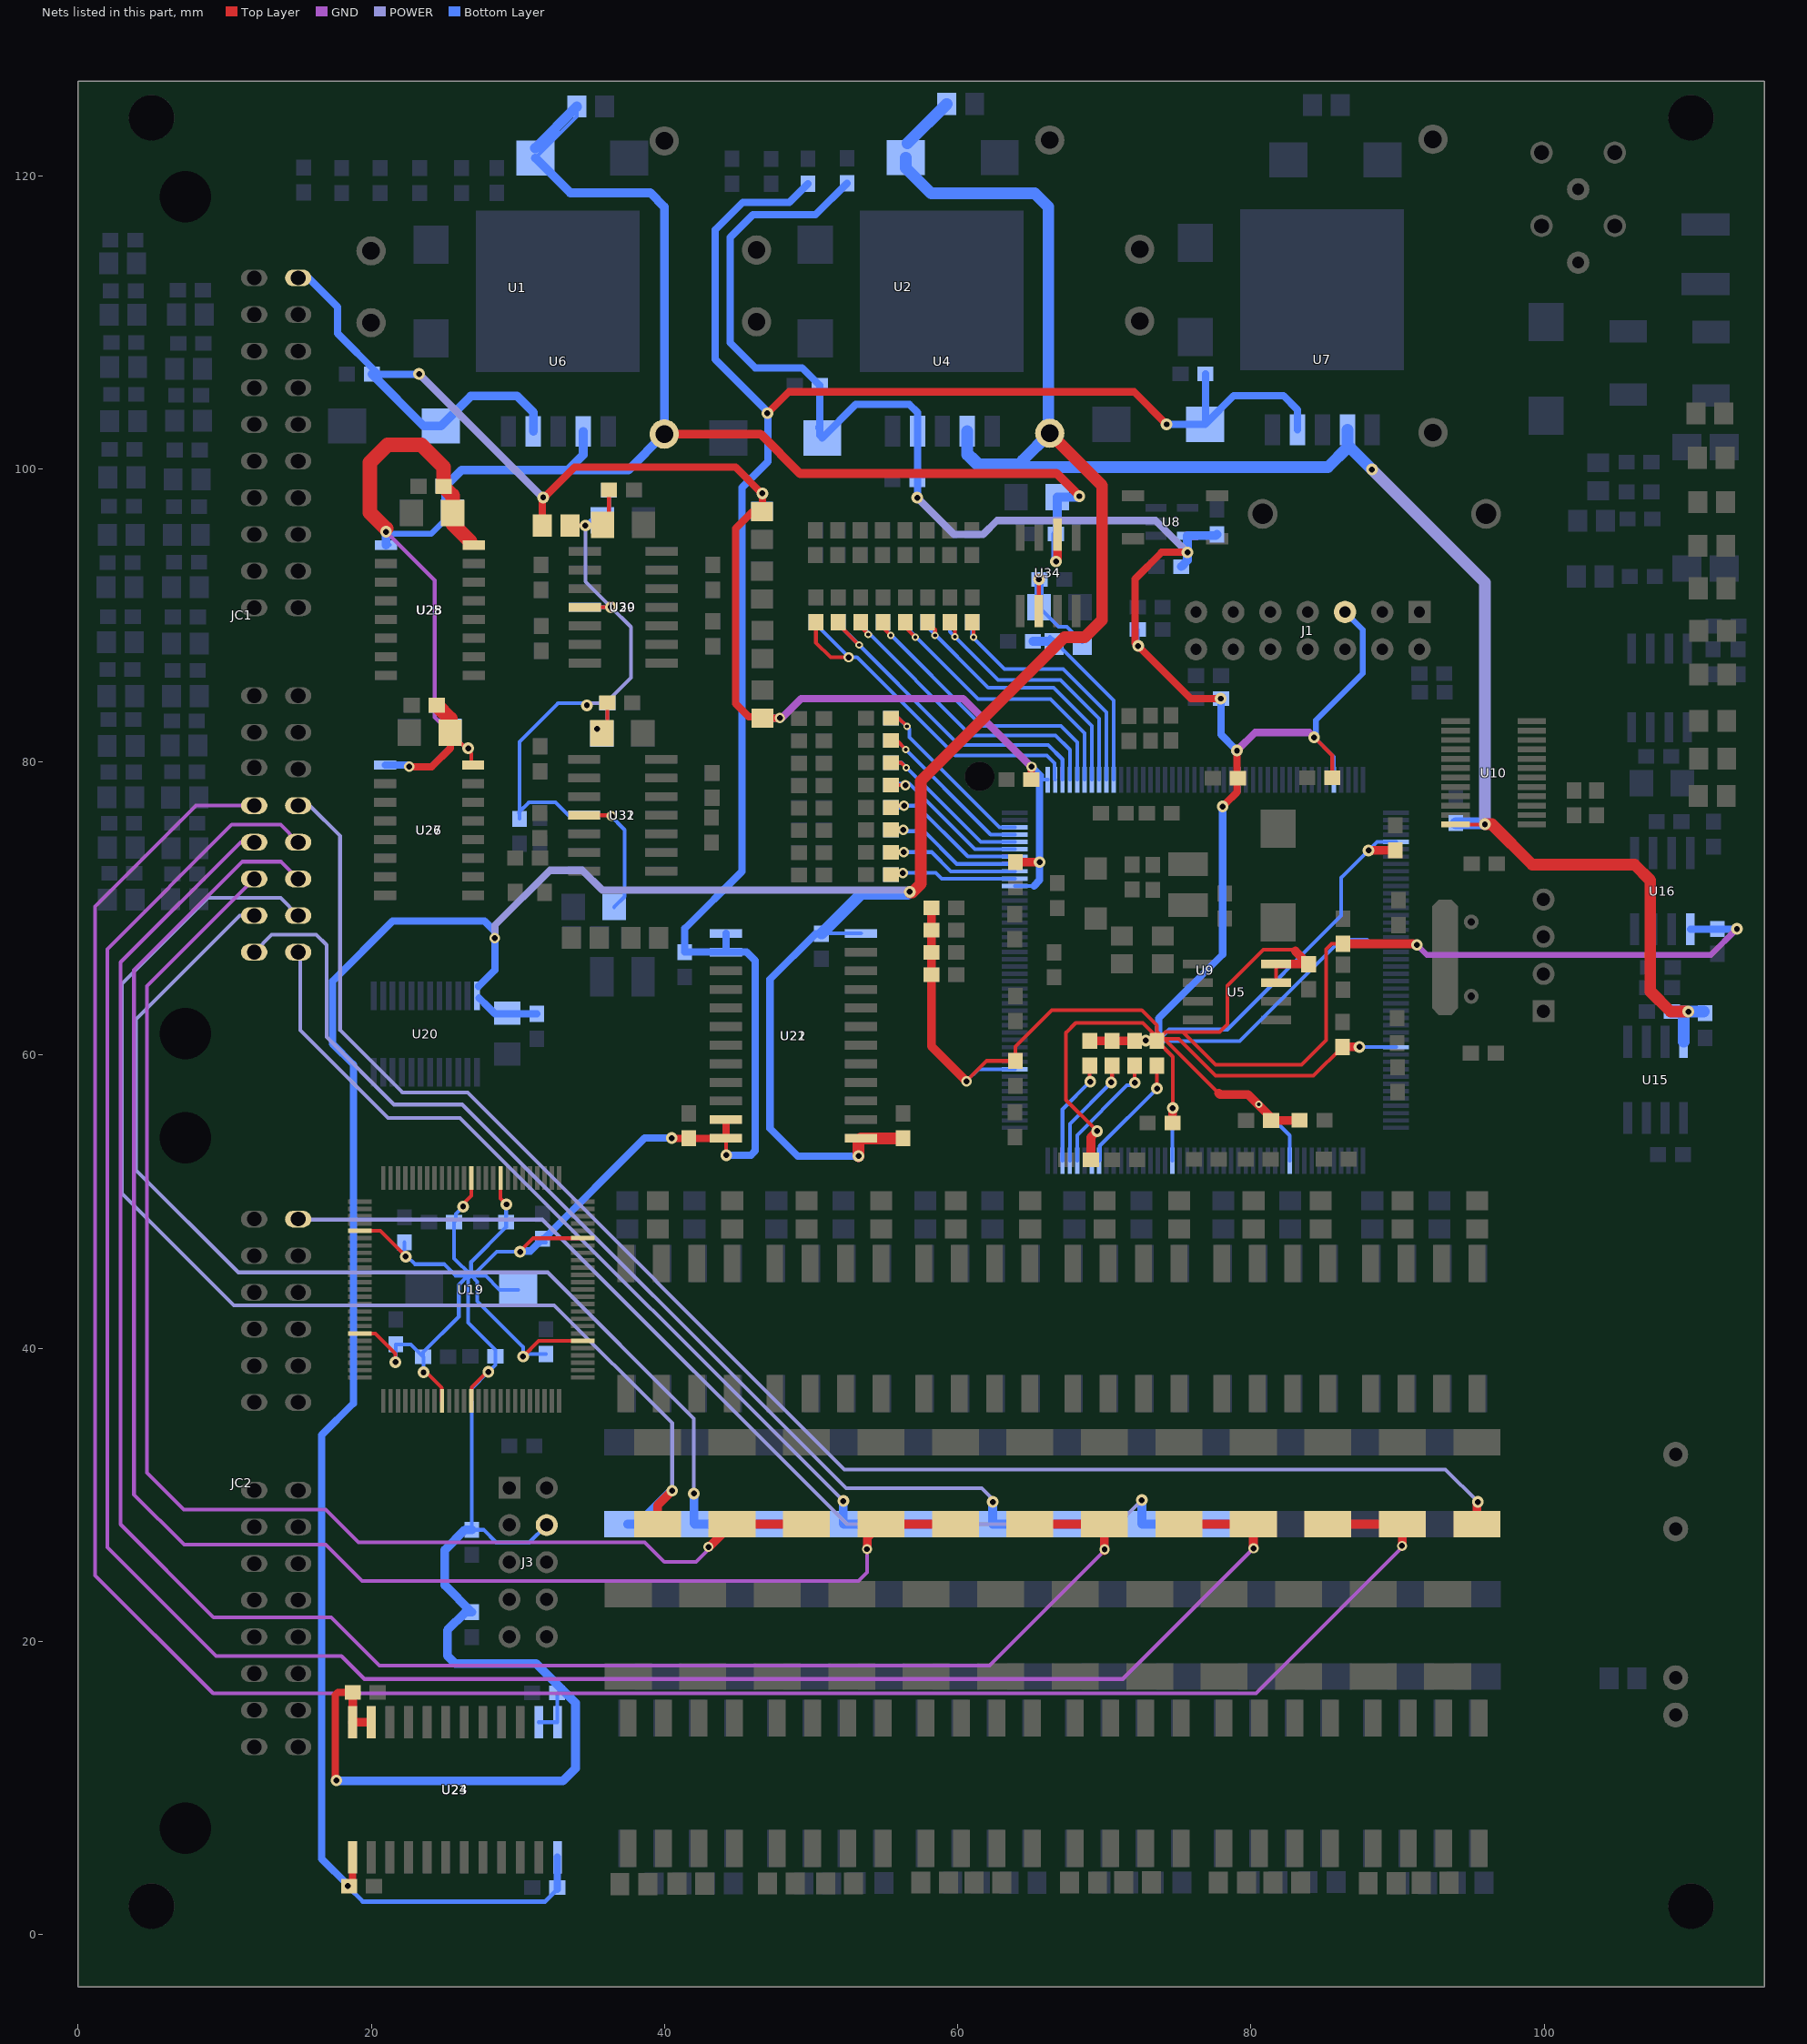
[diagram p0: the nets of this part, all layers, seen from the top]
# Altium PCB MISC86180.PCBDOC (part 4 of 9)
Units mm, origin at the board's own origin, x right, y up, seen from the top; angles counter-clockwise.
Board outline 115 x 130 mm, 4 copper layers (Top Layer, GND, POWER, Bottom Layer); 475 components, 355 nets, 1755 pads, 459 vias.

## Via types
v1: diameter 0.8, hole 0.4, Top Layer to Bottom Layer, 339 vias
v2: diameter 0.7, hole 0.4, Top Layer to Bottom Layer, 83 vias
v3: diameter 0.5, hole 0.254, Top Layer to Bottom Layer, 37 vias

## Nets (pads, with @x,y where several pads share a name; then routed paths per layer and width w, separated by ;. In a path a pad name is that pad's centre, name@x,y a point inside that pad or via, vN(x,y) a via of type N, cw(c..) or ccw(c..) an arc to the next point about the centre after c; other vN are vias at no path point) (continued)
+3.3VA: C15.1 C16.2 C125.2 C127.2 C201.2 C203.2 JC1.1 R131.1 R133.1 R136.1 U6.4 U9.34 U9.45 | length 111.7
  Top Layer w0.254: v1@46.65,98.3 v1(46.67,98.32)
  Top Layer w0.5: R136.1@31.661,96.126 31.661,97.911 33.86,100.11 44.84,100.11 v1@46.65,98.3 ; v1(46.67,98.32) 46.67,97.095 R133.1@46.65,97.075 46.005,97.075 44.85,95.92 44.85,83.97 45.736,83.084 46.604,83.084 R131.1@46.686,83.001 v2@47.949,83.001 ; C203.2@65.02,78.802 65.02,79.6 v2@65.06,79.64
  Top Layer w0.6: C201.2@63.918,73.168 v1(65.582,73.168)
  GND w0.5: v2(47.86,83.01) 47.89,82.98 47.97,82.98 49.31,84.32 60.36,84.32 65.02,79.66 v2@65.06,79.66
  POWER w0.5: v1(23.26,106.47) v1@31.69,98.04
  Bottom Layer w0.254: C127.2@46.65,97.093 46.65,98.3 v1(46.67,98.32) ; v2(47.86,83.01) 47.887,82.983 47.89,82.98 47.97,82.98 v2@47.967,82.983 ; U9.34@63.889,71.543 65.193,71.543 ; 65.582,78.755 65.62,78.793 U9.45@66.139,78.793
  Bottom Layer w0.5: JC1.1@15.01,113.022 15.718,113.022 17.7,111.04 17.7,109.23 20.472,106.458 v1@23.248,106.458 ; C125.2@46.686,82.983 47.887,82.983 v2@47.967,82.983 ; v2(65.03,79.67) 65.62,79.08 65.62,78.793 ; 65.193,71.543 65.582,71.932 v1(65.582,73.168) 65.582,78.755
  Bottom Layer w0.6: C16.2@20.04,106.458 23.576,102.922 C15.1@24.744,102.922 26.792,104.97 29.94,104.97 31.047,103.863 U6.4@31.047,102.555
  other v1: 31.72,98.04
+3.3VD: C11.1 C12.2 C19.2 C20.2 C21.2 C22.2 C23.2 C24.2 C25.2 C26.2 C27.2 C28.2 C29.2 C68.2 J1.5 R1.1 R2.1 R6.1 R7.1 R8.2 R9.2 R10.2 R11.2 R12.2 R86.1 R88.1 R90.1 R92.1 R94.1 U4.4 U5.3 U5.4 U8.5 U9.9 U9.71 U9.84 U9.93 U9.107 U9.121 U9.143 U9.159 U9.170 U16.1 | length 356.9
  Top Layer w0.254: v2(60.59,58.22) 61.98,59.61 C27.2@63.928,59.61 63.928,60.578 66.41,63.06 72.54,63.06 73.57,62.03 73.57,61.62 77.795,57.395 ; v1@69.39,54.71 v1(69.5,54.82) 67.38,56.94 67.38,61.53 68.04,62.19 72.61,62.19 R12.2@73.57,61.23 ; R10.2@70.522,60.976 R11.2@72.046,60.976 ; C20.2@74.64,55.372 C20.2@74.66,55.392 ; v1(74.66,56.39) 74.66,59.886 R12.2@73.57,60.976 73.582,60.988 R12.2@73.714,61.12 ; v1(79.04,80.78) v1@79.1,80.72 ; C22.2@81.36,55.542 81.36,55.56 C22.2@81.36,55.59 ; U5.3@81.713,64.94 U5.4@81.713,66.21 ; 83.024,67.104 82.938,67.19 80.83,67.19 78.38,64.74 78.38,62.1 77.85,61.57 75.35,61.57 ; R8.2@83.304,55.542 R8.2@83.31,55.548 ; C26.2@83.928,66.2 83.918,66.21 C26.2@84.1,66.21 ; v1(84.3,81.68) 85.54,80.44 C29.2@85.54,78.922 85.563,78.922 C29.2@85.64,78.999 ; C23.2@86.232,60.56 84.262,58.59 77.59,58.59 75.06,61.12 R12.2@73.714,61.12 ; C24.2@86.342,67.52 C24.2@86.262,67.6 85.49,67.6 85.12,67.23 85.12,61.02 83.44,59.34 77.58,59.34 75.35,61.57 ; v1@88.02,73.98 v1@88.15,73.98 ; v1@91.15,67.52 v1(91.31,67.52) ; R12.2@73.714,61.12 74.164,61.57 75.35,61.57 ; v1(78.06,76.96) 78.22,77.12 78.4,77.12 78.24,76.96 v1(78.06,76.96)
  Top Layer w0.5: v1(75.662,94.3) 73.9,94.3 72.09,92.49 72.09,88.12 v1(72.3,87.91) 75.888,84.322 v1(77.932,84.322) ; v1@78.22,77.12 79.04,77.94 v1(79.04,80.78)
  Top Layer w0.6: R92.1@58.2,70.054 R90.1@58.2,68.53 R88.1@58.2,67.006 R86.1@58.2,65.482 58.2,60.61 v2(60.59,58.22) ; R9.2@68.998,60.976 R10.2@70.522,60.976 R11.2@72.046,60.976 R12.2@73.57,60.976 ; C25.2@69.08,52.862 69.08,54.4 v1@69.39,54.71 ; C20.2@74.64,55.372 74.64,56.37 v1(74.66,56.39) ; 77.795,57.395 77.87,57.32 79.78,57.32 81.36,55.74 C22.2@81.36,55.59 ; C22.2@81.36,55.542 R8.2@83.304,55.542 ; U5.4@81.713,66.21 83.918,66.21 83.024,67.104 ; C23.2@86.232,60.56 v1(87.39,60.56) ; C24.2@86.262,67.6 91.07,67.6 v1@91.15,67.52 ; v1@88.15,73.98 C21.2@89.832,73.98
  GND w0.254: v1(79.04,80.78) 79.06,80.78 79.14,80.86 79.14,80.88 v1@79.14,80.93 ; v1@84.11,81.56 84.18,81.56 v1(84.3,81.68)
  GND w0.4: v1(91.31,67.52) 92,66.83 111.35,66.83 v1(113.14,68.62)
  GND w0.5: v1(79.04,80.78) 79.14,80.88 80.27,82.01 83.97,82.01 v1(84.3,81.68)
  POWER w0.5: v1(57.23,98.03) 59.74,95.52 61.726,95.52 62.676,96.47 73.492,96.47 v1(75.662,94.3)
  Bottom Layer w0.254: C11.1@50.404,102.742 C11.1@50.404,102.88 ; C11.1@50.58,102.276 C11.1@50.754,102.102 52.98,104.328 ; v2(60.59,58.22) 61.413,59.043 U9.9@63.889,59.043 ; U9.170@69.139,52.793 69.139,54.459 v1(69.5,54.82) ; v1@72.272,87.938 R6.1@72.272,89.032 ; 73.725,61.14 73.725,61.055 ; U9.159@74.639,52.793 v1@74.639,56.369 ; v1(77.932,84.322) R7.1@77.95,84.322 ; v1@78.894,80.714 79.139,80.469 U9.71@79.139,78.793 ; v3(80.52,56.64) 82.639,54.521 U9.143@82.639,52.793 ; v1@84.43,81.55 85.639,80.341 U9.84@85.639,78.793 U9.84@85.65,78.783 ; v1(87.39,60.56) 87.407,60.543 U9.121@89.889,60.543 ; U9.93@89.889,74.543 88.583,74.543 v1(88.01,73.97) 86.15,72.11 86.15,69.52 78.38,61.75 74.42,61.75 73.725,61.055 ; v1@91.287,67.543 U9.107@89.889,67.543 88.247,67.543 87.92,67.87 86.15,67.87 79.23,60.95 73.62,60.95 73.725,61.055
  Bottom Layer w0.4: v1@84.43,81.55 84.43,82.85 87.62,86.04 87.62,89.019 J1.5@86.406,90.233
  Bottom Layer w0.5: C11.1@50.58,102.276 C12.2@50.58,105.688 49.378,106.89 46.18,106.89 44.47,108.6 44.47,115.78 46.02,117.33 50.29,117.33 R94.1@52.442,119.482 ; C11.1@50.754,102.102 53.042,104.39 56.687,104.39 57.247,103.83 U4.4@57.247,102.565 v1@57.247,98.047 ; 73.725,61.14 73.69,61.175 73.69,62.5 78.06,66.87 v1(78.06,76.96) ; R7.1@77.95,84.322 77.95,81.87 78.894,80.926 v1@78.894,80.714 ; U16.1@109.963,68.591 v1@113.111,68.591
  Bottom Layer w0.6: v1(72.82,61) 73.515,61 73.69,61.175 ; R2.1@75.24,93.332 75.662,93.754 v1(75.662,94.3) U8.5@75.662,95.435 77.581,95.435 C19.2@77.672,95.526
+3.3VD2: C17.1 C18.2 C81.1 C82.2 C83.2 C84.2 C85.2 C86.2 C87.2 C88.2 C89.2 C92.2 C93.2 C94.2 C95.2 J3.4 R84.1 R85.1 R95.1 U7.4 U19.9 U19.13 U19.31 U19.45 U19.59 U19.63 U19.80 U19.94 U21.23 U21.24 U22.23 U22.24 U23.23 U23.24 U24.23 U24.24 | length 297.7
  Top Layer w0.254: v1@17.54,10.6 v1@17.54,10.735 ; v1@17.605,10.535 v1(17.62,10.52) ; 17.605,16.415 17.605,16.445 ; U23.24@18.719,14.492 U23.24@18.73,14.503 ; U19.94@19.216,41.014 20.276,41.014 21.64,39.65 v1(21.64,39.06) ; U19.80@19.216,48.014 20.606,48.014 22.34,46.28 v1(22.34,46.26) ; v1(23.56,38.36) 23.751,38.36 24.81,37.301 24.81,36.42 U19.9@24.816,36.414 ; v1(26.26,49.67) 26.1,49.67 26.092,49.678 26.092,49.68 26.816,50.404 U19.63@26.816,51.614 ; U19.13@26.816,36.414 26.861,36.459 26.861,37.34 27.911,38.39 v1(27.98,38.39) ; U19.59@28.816,51.614 28.816,50.214 v1(29.21,49.82) ; v1(30.15,46.58) 30.15,46.63 31.03,47.51 34.412,47.51 U19.45@34.416,47.514 ; v1(30.35,39.44) 31.42,40.51 34.412,40.51 U19.31@34.416,40.514 ; U22.24@44.192,54.329 U22.24@44.192,54.329 v1@44.192,53.198
  Top Layer w0.5: v1@17.54,10.6 v1@17.605,10.535 ; v1@17.54,10.735 17.54,16.35 17.605,16.415 17.718,16.528 C94.2@18.73,16.528 ; v1@40.5,54.33 C92.2@41.662,54.33 U22.24@44.192,54.329 ; U22.24@44.192,54.329 U22.23@44.192,55.599 ; v1(47.01,103.79) 48.47,105.25 72.02,105.25 v1(74.238,103.032)
  Top Layer w0.6: U23.24@18.719,14.492 U23.23@19.989,14.492 ; U23.24@18.73,14.503 C94.2@18.73,16.528
  Bottom Layer w0.254: v1(17.62,10.52) v1@17.69,10.59 ; v1(21.64,39.06) 21.658,39.078 C86.2@21.658,40.27 22.682,40.27 C88.2@23.53,39.422 ; C87.2@22.262,47.228 22.262,46.338 v1(22.34,46.26) 22.45,46.26 22.97,45.74 24.97,45.74 25.745,44.965 26.61,44.965 25.965,44.32 25.965,42.165 23.53,39.73 C88.2@23.53,39.422 ; v1(23.56,38.36) 23.56,39.392 C88.2@23.53,39.422 ; v1(26.26,49.67) 25.76,49.17 25.76,48.73 C89.2@25.634,48.604 25.634,46.136 26.805,44.965 ; v1(29.21,49.82) 29.19,49.8 C82.2@29.19,48.604 29.19,48.28 26.805,45.895 26.805,44.965 ; C81.1@30.01,43.996 28.75,43.996 27.781,44.965 26.95,44.965 ; v1@30.21,46.64 v1(30.15,46.58) 28.565,46.58 26.95,44.965 ; U24.23@31.419,14.492 U24.24@32.689,14.492 ; C84.2@31.678,47.228 C84.2@31.914,47.228 ; C84.2@31.678,47.47 C84.2@31.77,47.47 ; C85.2@31.914,39.608 30.518,39.608 v1(30.35,39.44) 30.35,40.09 27.22,43.22 27.22,44.55 26.805,44.965 ; J3.4@31.965,27.945 30.769,26.75 28.53,26.75 27.66,27.62 R84.1@26.848,27.62 26.848,37.258 v1(27.98,38.39) 28.46,38.87 C83.2@28.46,39.448 28.46,39.89 26.61,41.74 26.61,44.77 26.805,44.965 ; U24.24@32.66,14.521 U24.24@32.689,14.492 ; C95.2@32.689,16.459 U24.24@32.689,14.492 ; v1(44.21,53.18) v1@44.36,53.18 ; 26.805,44.965 26.95,44.965
  Bottom Layer w0.5: v1@30.04,46.64 30.21,46.64 30.848,46.64 C84.2@31.678,47.47 ; C84.2@31.77,47.47 38.64,54.34 v1(40.49,54.34) ; U21.23@44.192,67.029 C93.2@41.382,67.03 41.382,68.642 45.27,72.53 45.27,98.71 47.05,100.49 47.05,103.86 43.45,107.46 43.45,116.3 45.33,118.18 48.516,118.18 R95.1@49.788,119.452 ; U21.24@44.192,68.299 U21.23@44.192,67.029 45.591,67.029 46.18,66.44 46.18,53.47 45.89,53.18 v1@44.36,53.18 ; v1(74.238,103.032) C17.1@76.864,103.032 C17.1@76.89,103.058 ; C18.2@76.89,106.468 C17.1@76.89,103.058 ; U7.4@83.167,102.665 83.167,104.033 82.2,105 78.832,105 C17.1@76.89,103.058
  Bottom Layer w0.6: v1(17.62,10.52) 17.64,10.5 33.08,10.5 33.92,11.34 33.92,15.81 31.23,18.5 25.71,18.5 25.18,19.03 25.18,20.77 26.41,22 R85.1@26.848,22 25.01,23.838 25.01,26.24 26.39,27.62 R84.1@26.848,27.62
+5V: C6.1 C7.2 C57.2 C67.2 C90.2 C91.2 C96.2 C97.2 C98.2 C99.2 R21.2 U2.3 U4.2 U7.2 U10.24 U15.8 U20.24 U21.1 U22.1 U23.1 U24.1 | length 340.5
  Top Layer w0.254: v1(53.23,53.11) v1@53.392,53.272 ; 53.392,54.02 U22.1@53.392,54.329 ; U10.24@93.946,75.738 v1@95.938,75.738
  Top Layer w0.5: C98.2@18.48,3.308 18.725,3.553 U23.1@18.725,5.28
  Top Layer w0.8: v1(53.23,53.11) 53.23,54.02 ; U22.1@53.392,54.329 C96.2@56.272,54.33 ; v1(56.72,71.14) 56.77,71.09 56.88,71.09 57.474,71.684 57.474,78.704 67.277,88.507 68.653,88.507 69.84,89.694 69.84,98.858 U2.3@66.271,102.428 ; v1(95.95,75.75) 96.43,75.75 99.18,73 106.154,73 107.23,71.924 107.23,66.02 107.23,64.35 108.612,62.968 v1(109.83,62.968)
  POWER w0.254: v2(28.42,67.99) v2@28.42,68.18
  POWER w0.5: v2@28.42,68.18 28.42,68.85 32.18,72.61 34.4,72.61 35.75,71.26 56.47,71.26 56.637,71.093 56.673,71.093 v1(56.72,71.14)
  POWER w0.8: v1(88.25,99.95) 95.95,92.25 v1(95.95,75.75)
  Bottom Layer w0.254: C90.2@31.237,62.867 C90.2@31.288,62.816 ; C97.2@50.692,68.28 50.711,68.299 U21.1@53.392,68.299 ; C6.1@56.456,121.228 C6.1@56.559,121.331 ; 60.647,101.463 61.53,100.58 64.423,100.58 ; U2.3@66.25,102.522 66.25,102.448 U2.3@66.271,102.428 ; 86.407,101.597 86.567,101.757 U7.2@86.567,101.633 ; v1@95.87,75.83 v1(95.95,75.75) ; R21.2@110.874,62.968 R21.2@110.972,62.87
  Bottom Layer w0.3: v1@18.4,3.27 19.412,2.258 31.858,2.258 C99.2@32.68,3.08
  Bottom Layer w0.5: v1@18.4,3.27 v1(18.4,3.33) 18.4,3.39 16.62,5.17 16.62,34.09 18.77,36.24 18.77,59.36 17.36,60.77 17.36,65.04 21.46,69.14 27.72,69.14 28.42,68.44 v2(28.42,67.99) 28.42,65.8 27.32,64.7 U20.24@27.32,64.68 ; U20.24@27.36,63.889 27.97,63.28 28.129,63.12 28.433,62.816 C90.2@31.288,62.816 ; C99.2@32.68,3.08 C99.2@32.68,3.208 ; C99.2@32.68,3.228 32.68,5.283 U24.1@32.689,5.292 ; C97.2@50.692,68.28 50.3,68.28 47.19,65.17 47.19,55 49.08,53.11 v1(53.23,53.11)
  Bottom Layer w0.8: C97.2@50.711,68.299 53.422,71.01 56.59,71.01 v1(56.72,71.14) ; C6.1@56.456,121.228 56.456,120.514 58.18,118.79 65.25,118.79 66.176,117.864 U2.3@66.176,102.522 ; C6.1@56.559,122.2 C7.2@59.251,124.892 ; U4.2@60.647,102.565 60.647,101.463 60.647,100.953 61.49,100.11 85.24,100.11 86.567,101.437 86.567,101.633 v1(88.25,99.95) ; 64.423,100.58 U2.3@66.271,102.428 ; U7.2@86.567,101.757 U7.2@86.567,102.665 ; C57.2@93.968,75.83 v1@95.87,75.83 ; C67.2@108.7,62.968 v1(109.83,62.968) R21.2@110.874,62.968 ; U15.8@109.501,60.913 109.501,62.64
+5VA: C3.1 C4.2 C129.2 C130.2 C131.2 C140.2 C141.2 C142.2 C143.2 C144.2 C205.2 C206.2 U1.3 U6.2 U25.16 U26.16 U27.16 U28.16 U34.2 | length 153.7
  Top Layer w0.254: v2@22.5,79.651 v2@22.639,79.79 ; C141.2@24.77,83.75 C141.2@24.77,83.87 ; C129.2@24.92,97.611 C129.2@25.539,96.992 C129.2@25.539,96.251 ; C130.2@25.381,81.34 C130.2@25.381,82.006 26.81,80.577 26.81,79.911 U27.16@26.934,79.787 ; v1(66.7,93.68) v1@66.735,93.715
  Top Layer w0.5: v2(22.58,79.68) 24.12,79.68 25.381,80.941 C130.2@25.381,82.006
  Top Layer w0.6: U1.3@39.981,102.368 46.544,102.368 49.232,99.68 66.74,99.68 v1(68.29,98.13) ; v1@66.735,93.715 66.793,93.773 U34.2@66.793,95.507
  Top Layer w1: v1@21,95.917 19.91,97.007 19.91,100.43 21.12,101.64 23.4,101.64 24.92,100.12 C140.2@24.92,98.798 25.539,98.179 C129.2@25.539,96.992 25.539,96.251 U25.16@26.735,95.055 ; C141.2@24.46,83.872 25.381,82.951 C130.2@25.381,82.006
  GND w0.254: v1(21,95.7) 24.32,92.38 24.32,83.06 26.45,80.93 v1(26.61,80.93)
  Bottom Layer w0.254: U28.16@20.998,94.797 U28.16@21.257,94.797 ; v1@20.998,95.548 v1@21,95.55 ; v1@21.06,95.61 v1@21,95.55 ; v1@21.14,95.56 v1(21,95.7) v1@21,95.55 ; v2@22.58,79.79 22.63,79.79 24.05,79.79 25.381,81.121 C143.2@25.381,82.042 ; C143.2@24.77,82.653 C144.2@24.77,83.906 ; C3.1@31.186,121.208 34.021,124.043 C4.2@34.021,124.712 ; v1@66.69,93.69 v1(66.7,93.68) ; C205.2@66.779,98.068 C205.2@66.841,98.13 ; v1@68.228,98.13 v1(68.29,98.13)
  Bottom Layer w0.4: v1@21.14,95.56 24.081,95.56 C131.2@25.529,97.008
  Bottom Layer w0.5: U26.16@20.941,79.79 v2@22.58,79.79
  Bottom Layer w0.6: U28.16@20.998,94.797 20.998,95.548 v1@20.998,95.698 ; C131.2@25.529,97.008 25.074,97.463 25.074,98.834 26.148,99.908 33.398,99.908 ; C3.1@31.186,121.208 33.574,118.82 39.03,118.82 39.981,117.869 U1.3@39.981,102.368 37.522,99.908 33.398,99.908 ; U6.2@34.447,102.555 34.447,100.957 33.398,99.908 ; v1@66.69,93.69 C206.2@66.69,95.548 66.779,95.637 C205.2@66.779,98.068 v1@68.228,98.068
  Bottom Layer w0.7: C3.1@31.186,121.877 C4.2@34.021,124.712
+OPV: C132.2 C133.2 C134.2 C135.2 C136.2 C137.2 C138.2 C139.2 C208.2 C209.2 R136.2 U29.4 U30.4 U31.4 U32.4 | length 60.4
  Top Layer w0.254: R136.2@33.561,96.126 35.728,96.126 C132.2@35.765,96.162 36.204,96.601 C136.2@36.204,98.564 ; U31.4@34.514,76.365 36.325,76.365 v2(36.38,76.31) ; U29.4@34.554,90.551 v1@36.321,90.551 ; C134.2@35.725,81.976 36.094,82.345 C138.2@36.094,84.048
  POWER w0.254: v1(34.6,96.13) 34.6,92.31 v1(36.34,90.57) 37.7,89.21 37.7,85.76 35.96,84.02 34.83,84.02 34.7,83.89 v1(34.7,83.86)
  Bottom Layer w0.254: C209.2@30.092,76.5 30.092,76.585 30.747,77.24 32.55,77.24 33.415,76.375 U32.4@34.514,76.375 36.275,76.375 37.28,75.37 37.28,70.809 C208.2@36.569,70.098 ; C209.2@30.102,76.12 30.102,81.382 32.732,84.012 C139.2@36.094,84.012 36.094,82.309 C135.2@35.725,81.94 v1(35.4,82.265) ; U30.4@34.554,90.561 36.331,90.561 v1(36.34,90.57) ; v1(34.6,96.13) 34.952,96.482 C133.2@35.761,96.482 36.204,96.925 C137.2@36.204,98.528
A1_12: R12.1 U9.169 | length 8.1
  Top Layer w0.254: v1@73.57,57.73 R12.1@73.57,59.276
  Bottom Layer w0.254: U9.169@69.639,52.793 69.684,52.839 69.684,53.809 73.58,57.704 v1(73.58,57.72)
A1_13: R11.1 U9.172 | length 8.6
  Top Layer w0.254: v1@72.046,57.946 R11.1@72.046,59.276
  Bottom Layer w0.254: U9.172@68.139,52.793 68.139,54.539 71.54,57.94 72.04,57.94 72.07,57.97 v1(72.07,58.12)
A1_14: R10.1 U9.173 | length 7.8
  Top Layer w0.254: v1@70.522,57.982 R10.1@70.522,59.276
  Bottom Layer w0.254: U9.173@67.639,52.793 67.639,55.319 v1(70.46,58.14)
A1_15: R9.1 U9.174 | length 7.2
  Top Layer w0.254: v1@68.998,58.222 R9.1@68.998,59.276
  Bottom Layer w0.254: U9.174@67.139,52.793 67.139,56.299 v1(69.03,58.19)
AD_REF: C195.2 C196.2 R180.2 U34.6 | length 8
  Top Layer w0.254: U34.6@65.523,90.307 65.523,92.443 v1(65.53,92.45)
  Bottom Layer w0.254: C195.2@65.57,90.581 C195.2@65.541,90.552 66.877,89.215 67.422,89.215 R180.2@68.479,88.158 ; C196.2@65.57,92.413 C196.2@65.57,92.442
  Bottom Layer w0.6: C195.2@65.541,90.552 C196.2@65.541,92.413
AD_REFIN: C197.2 R180.1 U9.54 | length 12.8
  Bottom Layer w0.254: C197.2@65.107,88.12 C197.2@65.13,88.12 ; R180.1@66.292,88.538 70.639,84.191 U9.54@70.639,78.793
  Bottom Layer w0.6: C197.2@65.13,88.228 R180.1@66.389,88.228
ADCINA0: C171.2 R154.1 U9.42 | length 13.2
  Top Layer w0.254: R154.1@55.468,82.988 R154.1@55.44,82.988 55.962,82.988 v3(56.53,82.42)
  Bottom Layer w0.254: C171.2@55.44,82.988 55.952,82.988 56.7,82.24 56.7,81.69 62.847,75.543 U9.42@63.889,75.543
ADCINA1: C174.2 R156.1 U9.41 | length 12.5
  Top Layer w0.254: R156.1@55.536,81.464 R156.1@55.44,81.464 55.846,81.464 v3(56.46,80.85)
  Bottom Layer w0.254: C174.2@55.44,81.464 55.816,81.464 62.237,75.043 U9.41@63.889,75.043
ADCINA2: C177.2 R158.1 U9.40 | length 11.9
  Top Layer w0.254: R158.1@55.44,79.94 56.13,79.94 v3(56.47,79.6)
  Bottom Layer w0.254: C177.2@55.44,79.94 56.18,79.94 61.577,74.543 U9.40@63.889,74.543
ADCINA3: C180.2 R160.1 U9.39 | length 11.4
  Top Layer w0.254: R160.1@55.44,78.416 v2(56.424,78.416)
  GND w0.254: v2(56.424,78.416) v2@56.47,78.37
  Bottom Layer w0.254: C180.2@55.44,78.416 55.544,78.52 56.7,78.52 61.177,74.043 U9.39@63.889,74.043
ADCINA4: C183.2 R162.1 U9.38 | length 10.9
  Top Layer w0.254: R162.1@55.44,76.892 55.56,77.012 v2(56.33,77.012)
  Bottom Layer w0.254: C183.2@55.44,76.892 56.21,76.892 v2(56.33,77.012) 57.218,77.012 60.687,73.543 U9.38@63.889,73.543
ADCINA5: C186.2 R164.1 U9.37 | length 10.1
  Top Layer w0.254: R164.1@55.44,75.368 v2(56.282,75.368)
  Bottom Layer w0.254: C186.2@55.528,75.28 57.7,75.28 59.937,73.043 U9.37@63.889,73.043
ADCINA6: C189.2 R166.1 U9.36 | length 9.9
  Top Layer w0.254: R166.1@55.44,73.844 56.304,73.844 v2(56.31,73.85)
  Bottom Layer w0.254: C189.2@55.44,73.844 56.304,73.844 v2(56.31,73.85) 58.22,73.85 59.527,72.543 U9.36@63.889,72.543
ADCINA7: C192.2 R168.1 U9.35 | length 9.5
  Top Layer w0.254: R168.1@55.44,72.32 56.14,72.32 v2(56.25,72.43)
  Bottom Layer w0.254: C192.2@55.44,72.32 C192.2@55.47,72.29 ; C192.2@55.44,72.43 58.51,72.43 58.897,72.043 U9.35@63.889,72.043
ADCINB0: C147.2 R138.1 U9.46 | length 25.5
  Top Layer w0.254: R138.1@50.32,89.532 50.32,88.14 51.32,87.14 v2(52.55,87.14)
  Bottom Layer w0.254: C147.2@50.32,89.532 50.32,89.402 52.569,87.153 53.117,87.153 59.82,80.45 66.06,80.45 66.594,79.916 66.594,78.839 U9.46@66.639,78.793
ADCINB1: C150.2 R140.1 U9.47 | length 22.8
  Top Layer w0.254: R140.1@51.844,89.532 51.844,89.402 53.266,87.98 v3(53.27,87.98)
  Bottom Layer w0.254: C150.2@51.844,89.532 51.844,89.406 60.09,81.16 66.16,81.16 67.139,80.181 U9.47@67.139,78.793
ADCINB2: C153.2 R142.1 U9.48 | length 21.1
  Top Layer w0.254: R142.1@53.368,89.532 53.368,89.232 53.9,88.7 v3(53.89,88.69)
  Top Layer w0.6: R142.1@53.368,89.468 R142.1@53.368,89.532
  Bottom Layer w0.254: C153.2@53.368,89.532 53.368,89.352 60.9,81.82 66.65,81.82 67.639,80.831 U9.48@67.639,78.793
ADCINB3: C156.2 R144.1 U9.49 | length 20.5
  Top Layer w0.254: R144.1@54.892,89.532 54.892,89.168 v3(55.43,88.63)
  Bottom Layer w0.254: C156.2@54.892,89.532 54.892,89.208 61.64,82.46 67.02,82.46 68.139,81.341 U9.49@68.139,78.793
ADCINB4: C159.2 R146.1 U9.50 | length 20
  Top Layer w0.254: R146.1@56.416,89.528 R146.1@56.416,89.532 56.416,89.194 v3(57.1,88.51)
  Top Layer w0.6: R146.1@56.414,89.53 R146.1@56.416,89.532
  Bottom Layer w0.254: C159.2@56.416,89.532 56.416,89.254 v3@57.12,88.55 ; v3@57.11,88.56 v3@57.12,88.55 ; U9.50@68.639,78.793 68.639,81.971 66.32,84.29 61.38,84.29 v3@57.12,88.55
ADCINB5: C162.2 R148.1 U9.51 | length 19.1
  Top Layer w0.254: R148.1@57.94,89.532 58.45,89.022 v3(58.45,88.63)
  Bottom Layer w0.254: C162.2@57.94,89.532 57.94,89.21 62.08,85.07 66.54,85.07 69.139,82.471 U9.51@69.139,78.793
ADCINB6: C165.2 R150.1 U9.52 | length 18.6
  Top Layer w0.254: R150.1@59.464,89.532 59.81,89.186 v3(59.81,88.54)
  Top Layer w0.6: R150.1@59.464,89.532 R150.1@59.464,89.564
  Bottom Layer w0.254: C165.2@59.464,89.532 59.464,88.896 62.76,85.6 67,85.6 69.639,82.961 U9.52@69.639,78.793
ADCINB7: C168.2 R152.1 U9.53 | length 18
  Top Layer w0.254: R152.1@60.988,89.532 61.08,89.44 v3(61.08,88.51)
  Top Layer w0.6: R152.1@60.988,89.482 R152.1@60.988,89.532
  Bottom Layer w0.254: C168.2@60.988,89.532 60.988,88.542 63.18,86.35 67.19,86.35 70.139,83.401 U9.53@70.139,78.793
  Bottom Layer w0.6: C168.2@60.966,89.51 C168.2@60.988,89.532
BAT1: F1.1 JC1.24 | length 109.4
  Top Layer w0.6: F1.1@95.396,28.006 95.396,29.446 v1(95.47,29.52)
  POWER w0.254: JC1.24@15.01,77.022 15.788,77.022 17.87,74.94 17.87,61.69 22.12,57.44 26.56,57.44 52.27,31.73 93.26,31.73 v1(95.47,29.52)
BAT2: F2.1 F3.1 JC1.32 | length 162.6
  Top Layer w0.6: F3.1@85.236,28.006 F2.1@90.316,28.006 90.316,26.526 90.31,26.52 v2(90.3,26.52)
  GND w0.254: JC1.32@12.01,77.022 8.052,77.022 1.17,70.14 1.17,24.51 9.21,16.47 80.33,16.47 90.32,26.46 90.32,26.5 v2(90.3,26.52)
BAT3: F4.1 F5.1 JC1.25 | length 150.1
  Top Layer w0.6: F5.1@75.076,28.006 F4.1@80.156,28.006 80.156,26.384 v2(80.18,26.36)
  GND w0.254: JC1.25@15.01,74.522 13.812,75.72 10.48,75.72 1.99,67.23 1.99,26.43 9.4,19.02 17.96,19.02 19.54,17.44 71.24,17.44 v2@80.115,26.315
BAT4: F6.1 F7.1 JC1.33 | length 132.6
  Top Layer w0.254: F6.1@69.99,28 F6.1@69.996,28.006 ; v2@70.002,26.208 70.002,26.036 70.012,26.046 70.012,26.278 v2(70.01,26.28)
  Top Layer w0.6: F7.1@64.916,28.006 F6.1@69.996,28.006 69.996,26.214 v2@70.002,26.208
  GND w0.254: JC1.33@12.01,74.522 11.082,74.522 2.9,66.34 2.9,27.99 9.24,21.65 17.27,21.65 20.56,18.36 62.16,18.36 70.02,26.22 70.02,26.27 v2(70.01,26.28)
BAT5: F8.1 F9.1 JC1.26 | length 112
  Top Layer w0.6: v2(53.81,26.3) 53.812,26.298 53.816,26.298 53.82,26.302 53.82,27.07 F9.1@54.756,28.006 F8.1@59.836,28.006
  GND w0.254: JC1.26@15.01,72.022 13.832,73.2 11.21,73.2 3.81,65.8 3.81,30.02 7.23,26.6 16.9,26.6 19.377,24.123 53.233,24.123 53.82,24.71 53.82,26.29 v2(53.81,26.3)
BAT6: F10.1 F11.1 JC1.34 | length 93.1
  Top Layer w0.254: v2(42.99,26.45) v2@42.99,26.616 ; v2@42.99,26.3 v2(42.99,26.45) v2@42.99,26.616
  Top Layer w0.6: v2(42.99,26.45) 43.04,26.45 F11.1@44.596,28.006 F10.1@49.676,28.006
  GND w0.254: JC1.34@12.01,72.022 4.7,64.712 4.7,31.52 7.22,29 16.9,29 19.132,26.768 32.53,26.768 ; 32.892,26.768 32.53,26.768 ; v2(42.99,26.45) 42.99,26.27 42.14,25.42 39.989,25.42 38.64,26.768 32.53,26.768
BAT7: F12.1 F13.1 JC1.27 | length 84.5
  Top Layer w0.6: F12.1@39.516,28.006 39.516,29.286 v1(40.52,30.29)
  POWER w0.254: JC1.27@15.01,69.522 13.812,70.72 8.85,70.72 2.99,64.86 2.99,50.57 10.622,42.938 32.472,42.938 40.52,34.89 v1(40.52,30.29)
  Bottom Layer w0.254: v1@40.46,30.29 v1(40.52,30.29)
  Bottom Layer w0.6: F13.1@37.484,28.006 38.176,28.006 v1@40.46,30.29
BAT8: F14.1 F15.1 JC1.35 | length 79.2
  POWER w0.254: JC1.35@12.01,69.522 11.022,69.522 3.96,62.46 3.96,52.16 10.94,45.18 32.02,45.18 42,35.2 v1(42,30.09)
  Bottom Layer w0.254: v1(42,30.09) v1@42.056,30.034
  Bottom Layer w0.6: v1(42,30.09) 42,28.062 F14.1@42.056,28.006 F15.1@47.644,28.006
BAT9: F16.1 F17.1 JC1.28 | length 62.9
  POWER w0.254: JC1.28@15.01,67.022 15.16,66.872 15.16,61.71 21.15,55.72 26.05,55.72 v1(52.19,29.58)
  Bottom Layer w0.254: v1(52.19,29.58) v1@52.216,29.554
  Bottom Layer w0.6: v1(52.19,29.58) 52.19,28.032 F16.1@52.216,28.006 F17.1@57.804,28.006
BAT10: F18.1 F19.1 JC1.36 | length 77.8
  POWER w0.254: JC1.36@12.01,67.022 13.208,68.22 16.25,68.22 16.95,67.52 16.95,61.23 21.55,56.63 26.21,56.63 52.38,30.46 61.62,30.46 62.38,29.7 v1(62.38,29.52)
  Bottom Layer w0.254: v1@62.376,29.516 v1(62.38,29.52) ; F19.1@67.96,28.006 F19.1@67.964,28.006
  Bottom Layer w0.6: v1(62.38,29.52) 62.38,28.01 F19.1@67.96,28.01
BAT11: F20.1 F21.1 JC2.3 | length 74.1
  POWER w0.254: JC2.3@15.01,48.814 15.044,48.78 31.67,48.78 52.44,28.01 70.92,28.01 v1(72.55,29.64)
  Bottom Layer w0.254: v1@72.536,29.626 v1(72.55,29.64)
  Bottom Layer w0.6: v1(72.55,29.64) 72.55,28.02 72.564,28.006 F21.1@78.124,28.006